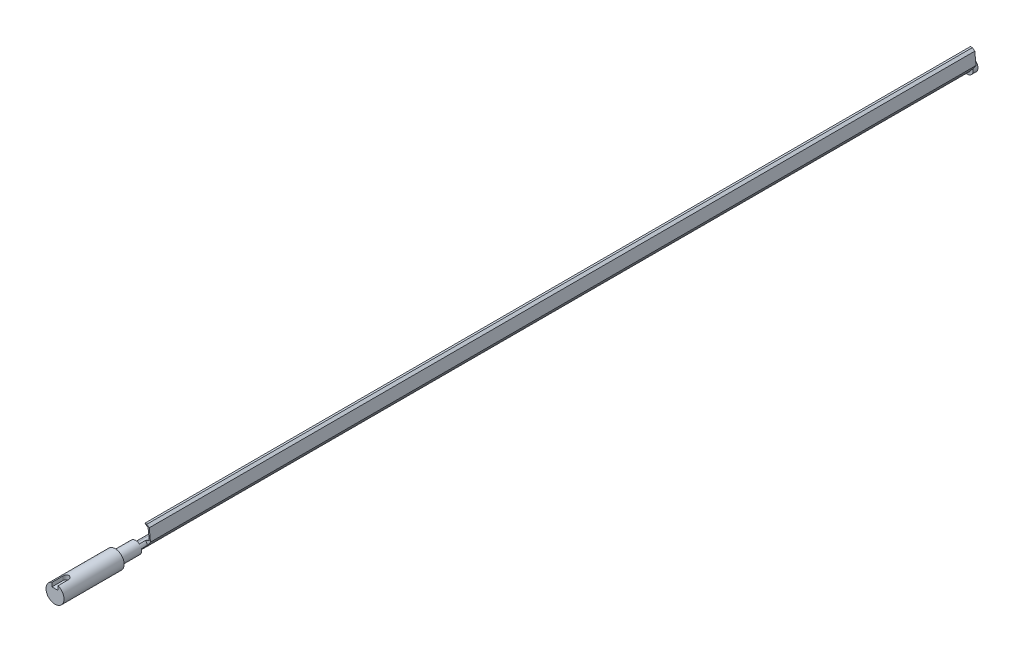
SolidWorks part; units mm, degrees
ref_plane "Front Plane" through (0, 0, 0) normal (0, 0, 1) x (1, 0, 0)
ref_plane "Top Plane" through (0, 0, 0) normal (0, 1, 0) x (1, 0, 0)
ref_plane "Right Plane" through (0, 0, 0) normal (1, 0, 0) x (0, 0, -1)
sketch "Sketch1" plane through (0, 0, 0) normal (0, 0, 1) x (1, 0, 0)
  circle A0 centre (0, 0) radius 100
  dimension "D1" = 200
extrude "Boss-Extrude1" add sketch "Sketch1" along normal blind 340
sketch "Sketch2" plane through (0, 0, 0) normal (0, 0, -1) x (-1, 0, 0)
  line L0 (-96.2334, 27.187) -> (-146.4287, 97.202)
  line L1 (-146.4287, 97.202) -> (-127.2387, 294.9434)
  line L2 (-127.2387, 294.9434) -> (-85.8554, 324.612)
  line L3 (-85.8554, 324.612) -> (-53.8157, 324.612)
  line L4 (-53.8157, 324.612) -> (-69.8355, 313.127)
  line L5 (-69.8355, 313.127) -> (-106.547, 286.8077)
  line L6 (-106.547, 286.8077) -> (-127.2387, 110.9598)
  line L7 (-127.2387, 110.9598) -> (-61.8256, 78.5977)
  line L8 (-61.8256, 78.5977) -> (0, 58.675)
  line L9 (-96.2334, 27.187) -> (-48.1874, -33.4774)
  circle A0 centre (0, 0) radius 100 construction
  arc A1 (-48.1874, -33.4774) -> (0, 58.675) centre (0, 0) ccw
extrude "Boss-Extrude2" add sketch "Sketch2" along normal blind 13824
sketch "Sketch3" plane through (0, 0, -13824) normal (0, 0, -1) x (-1, 0, 0)
  circle A0 centre (0, 0) radius 100
  dimension "D1" = 200
extrude "Boss-Extrude3" add sketch "Sketch3" along normal blind 80
sketch "Sketch4" plane through (0, 0, 0) normal (0, 0, 1) x (1, 0, 0)
  line L7 (96.2334, 27.187) -> (146.4287, 97.202)
  line L8 (146.4287, 97.202) -> (127.2387, 294.9434)
  line L9 (127.2387, 294.9434) -> (85.8554, 324.612)
  line L10 (85.8554, 324.612) -> (53.8157, 324.612)
  line L11 (53.8157, 324.612) -> (106.547, 286.8077)
  line L12 (106.547, 286.8077) -> (127.2387, 110.9598)
  line L13 (127.2387, 110.9598) -> (61.8256, 78.5977)
  line L14 (96.2334, 27.187) -> (146.4287, 97.202)
  line L15 (146.4287, 97.202) -> (127.2387, 294.9434)
  line L16 (127.2387, 294.9434) -> (85.8554, 324.612)
  line L17 (85.8554, 324.612) -> (53.8157, 324.612)
  line L18 (53.8157, 324.612) -> (106.547, 286.8077)
  line L19 (106.547, 286.8077) -> (127.2387, 110.9598)
  line L20 (127.2387, 110.9598) -> (61.8256, 78.5977)
  arc A1 (96.2334, 27.187) -> (61.8256, 78.5977) centre (0, 0) ccw
  arc A2 (96.2334, 27.187) -> (61.8256, 78.5977) centre (0, 0) ccw
  dimension "D1" = 0
extrude "Cut-Extrude1" cut sketch "Sketch4" against normal blind 100
sketch "Sketch6" plane through (0, 0, 340) normal (0, 0, 1) x (1, 0, 0)
  circle A0 centre (0, 0) radius 150
  dimension "D1" = 300
extrude "Boss-Extrude5" add sketch "Sketch6" along normal blind 1000
sketch "Sketch7" plane through (0, 0, 0) normal (0, 1, 0) x (1, 0, 0)
  line L0 (0, -1160) -> (0, -1460) construction
  line L1 (50, -1160) -> (50, -1460)
  line L2 (-50, -1160) -> (-50, -1460)
  line L4 (-150, -1340) -> (150, -1340) construction
  arc A0 (50, -1160) -> (-50, -1160) centre (0, -1160) ccw
  arc A1 (-50, -1460) -> (50, -1460) centre (0, -1460) ccw
  point P2 (0, -1310)
  dimension "D1" = 50
  dimension "D2" = 50
  dimension "D3" = 300
  dimension "D4" = 180
extrude "Cut-Extrude2" cut sketch "Sketch7" along normal blind 326
sketch "Sketch8" plane through (0, 0, 0) normal (0, 1, 0) x (1, 0, 0)
  line L2 (-50, -1160) -> (-50, -1340)
  line L3 (50, -1340) -> (50, -1160)
  line L4 (-50, -1160) -> (-50, -1340)
  line L5 (50, -1340) -> (50, -1160)
  line L7 (-50, -1340) -> (50, -1340)
  line L8 (-50, -1340) -> (50, -1340)
  arc A2 (50, -1160) -> (-50, -1160) centre (0, -1160) ccw
  arc A4 (50, -1160) -> (-50, -1160) centre (0, -1160) ccw
  dimension "D1" = 0
extrude "Boss-Extrude6" add sketch "Sketch8" along normal blind 75
